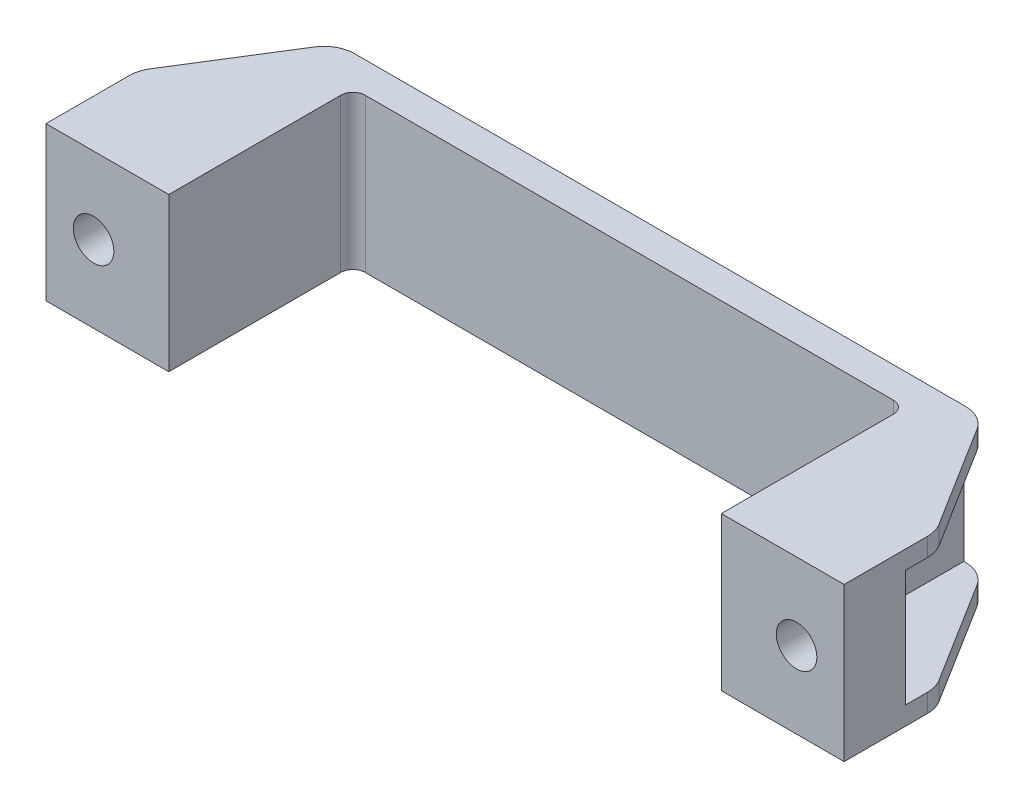
from build123d import *

# Parameters (mm, degrees)
BOSS_EXTRUDE1_DEPTH                               = 25
SKETCH2_W                                         = 18.5
SKETCH2_H                                         = 19
CUT_EXTRUDE1_DEPTH                                = 25
COUNTERBORE_FOR_PAN_HEAD_SCREW_OF_M61_D           = 6.6
COUNTERBORE_FOR_PAN_HEAD_SCREW_OF_M61_CBORE_D     = 13
COUNTERBORE_FOR_PAN_HEAD_SCREW_OF_M61_CBORE_DEPTH = 4.6
FILETE1_R                                         = 5
FILETE2_R                                         = 2


with BuildPart() as part:
    # Sketch1 → Boss-Extrude1 (new body)
    with BuildSketch(Plane(origin=(0, 0, 0), x_dir=(1, 0, 0), z_dir=(0, 1, 0))):
        Polygon((-52.5, 0), (52.5, 0), (65, -20), (65, -35), (45, -35), (45, -5), (-45, -5), (-45, -35), (-65, -35), (-65, -20), align=None)
    extrude(amount=BOSS_EXTRUDE1_DEPTH)

    # Sketch2 → Cut-Extrude1 (cut)
    with BuildSketch(Plane(origin=(0, 0, 0), x_dir=(-1, 0, 0), z_dir=(0, 0, -1))):
        with Locations((-58.75, 12.5)):
            Rectangle(SKETCH2_W, SKETCH2_H)
        with Locations((58.75, 12.5)):
            Rectangle(SKETCH2_W, SKETCH2_H)
    extrude(amount=-CUT_EXTRUDE1_DEPTH, mode=Mode.SUBTRACT)

    # Counterbore for pan head screw of M61 (through all)
    with Locations(Plane(origin=(0, 0, 25), x_dir=(-1, 0, 0), z_dir=(0, 0, -1))):
        with Locations((-57.25, 12.5), (57.25, 12.5)):
            CounterBoreHole(COUNTERBORE_FOR_PAN_HEAD_SCREW_OF_M61_D / 2, COUNTERBORE_FOR_PAN_HEAD_SCREW_OF_M61_CBORE_D / 2, COUNTERBORE_FOR_PAN_HEAD_SCREW_OF_M61_CBORE_DEPTH)

    # Filete1
    filete1_edges = [part.edges().sort_by_distance(p)[0] for p in [
        (-52.5, 23.5, 0),
        (52.5, 23.5, 0),
        (65, 23.5, 20),
        (-65, 23.5, 20),
        (52.5, 1.5, 0),
        (65, 1.5, 20),
        (-52.5, 1.5, 0),
        (-65, 1.5, 20),
    ]]
    fillet(filete1_edges, radius=FILETE1_R)

    # Filete2
    filete2_edges = [part.edges().sort_by_distance(p)[0] for p in [
        (45, 12.5, 5),
        (-45, 12.5, 5),
    ]]
    fillet(filete2_edges, radius=FILETE2_R)


solid = part.part
